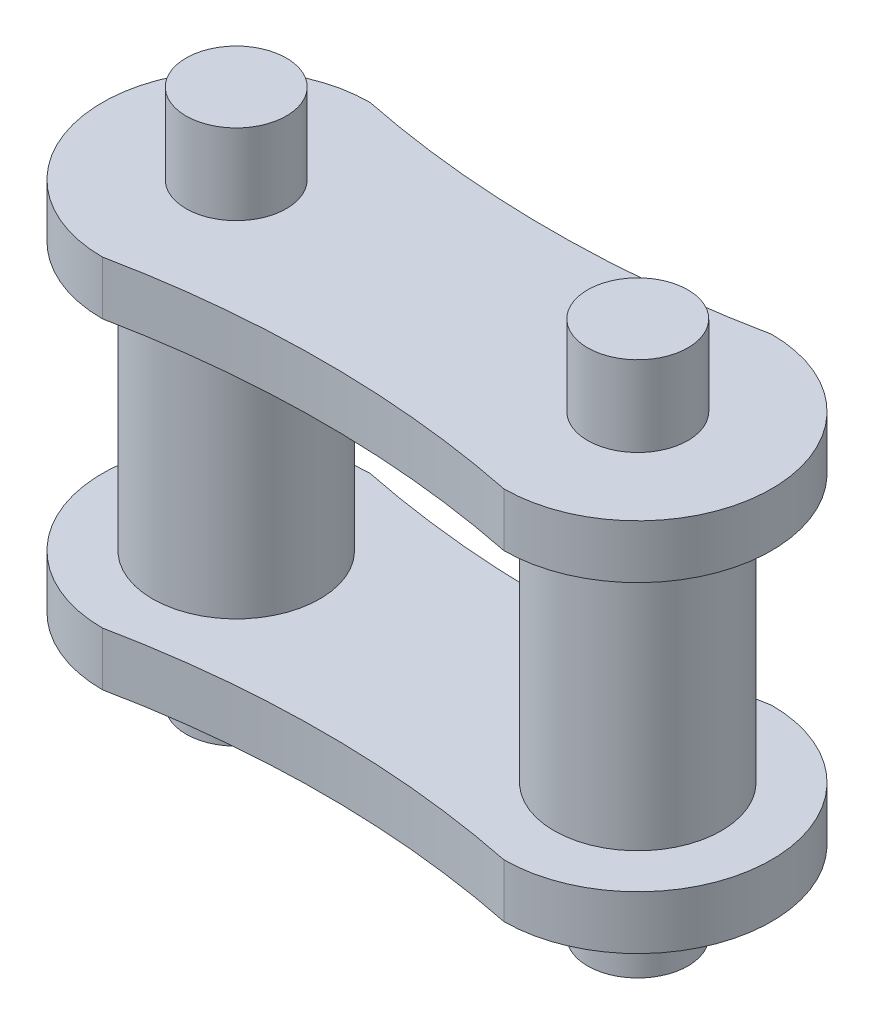
SolidWorks part; units mm, degrees
ref_plane "Front Plane" through (0, 0, 0) normal (0, 0, 1) x (1, 0, 0)
ref_plane "Top Plane" through (0, 0, 0) normal (0, 1, 0) x (1, 0, 0)
ref_plane "Right Plane" through (0, 0, 0) normal (1, 0, 0) x (0, 0, -1)
other "Configuration Table"
sketch "Sketch1" plane through (0, 0, 0) normal (0, 1, 0) x (1, 0, 0)
  line L0 (0, 0) -> (60, 0) construction
  arc A0 (0, 20) -> (0, -20) centre (0, 0) ccw
  arc A1 (60, -20) -> (60, 20) centre (60, 0) ccw
  arc A2 (0, 20) -> (60, 20) centre (30, 166.9694) ccw
  arc A3 (0, -20) -> (60, -20) centre (30, -166.9694) cw
  point P3 (30, 0)
  dimension "D2" = 20
  dimension "D3" = 150
  dimension "D4" = 150
  dimension "D1" = 60
extrude "Boss-Extrude1" add sketch "Sketch1" along normal blind 8
sketch "Sketch2" plane through (0, 8, 0) normal (0, 1, 0) x (1, 0, 0)
  circle A0 centre (0, 0) radius 12.5
  circle A1 centre (60, 0) radius 12.5
  dimension "D1" = 25
  dimension "D2" = 25
extrude "Boss-Extrude2" add sketch "Sketch2" along normal blind 40
pattern_linear "LPattern1" count 2 spacing 48 along (0, 1, 0) of "Boss-Extrude1"
sketch "Sketch3" plane through (0, 56, 0) normal (0, 1, 0) x (1, 0, 0)
  circle A0 centre (0, 0) radius 7.5
  circle A1 centre (60, 0) radius 7.5
  dimension "D1" = 15
  dimension "D2" = 15
extrude "Boss-Extrude3" add sketch "Sketch3" along normal blind 12
pattern_linear "LPattern2" count 2 spacing 68 along (0, -1, 0) of "Boss-Extrude3"
ref_point "Point1"
ref_point "Point2"
ref_plane "Plane1" through (0, 28, 0) normal (0, 1, 0) x (1, 0, 0)
equation "\"150、\"=151.54"
